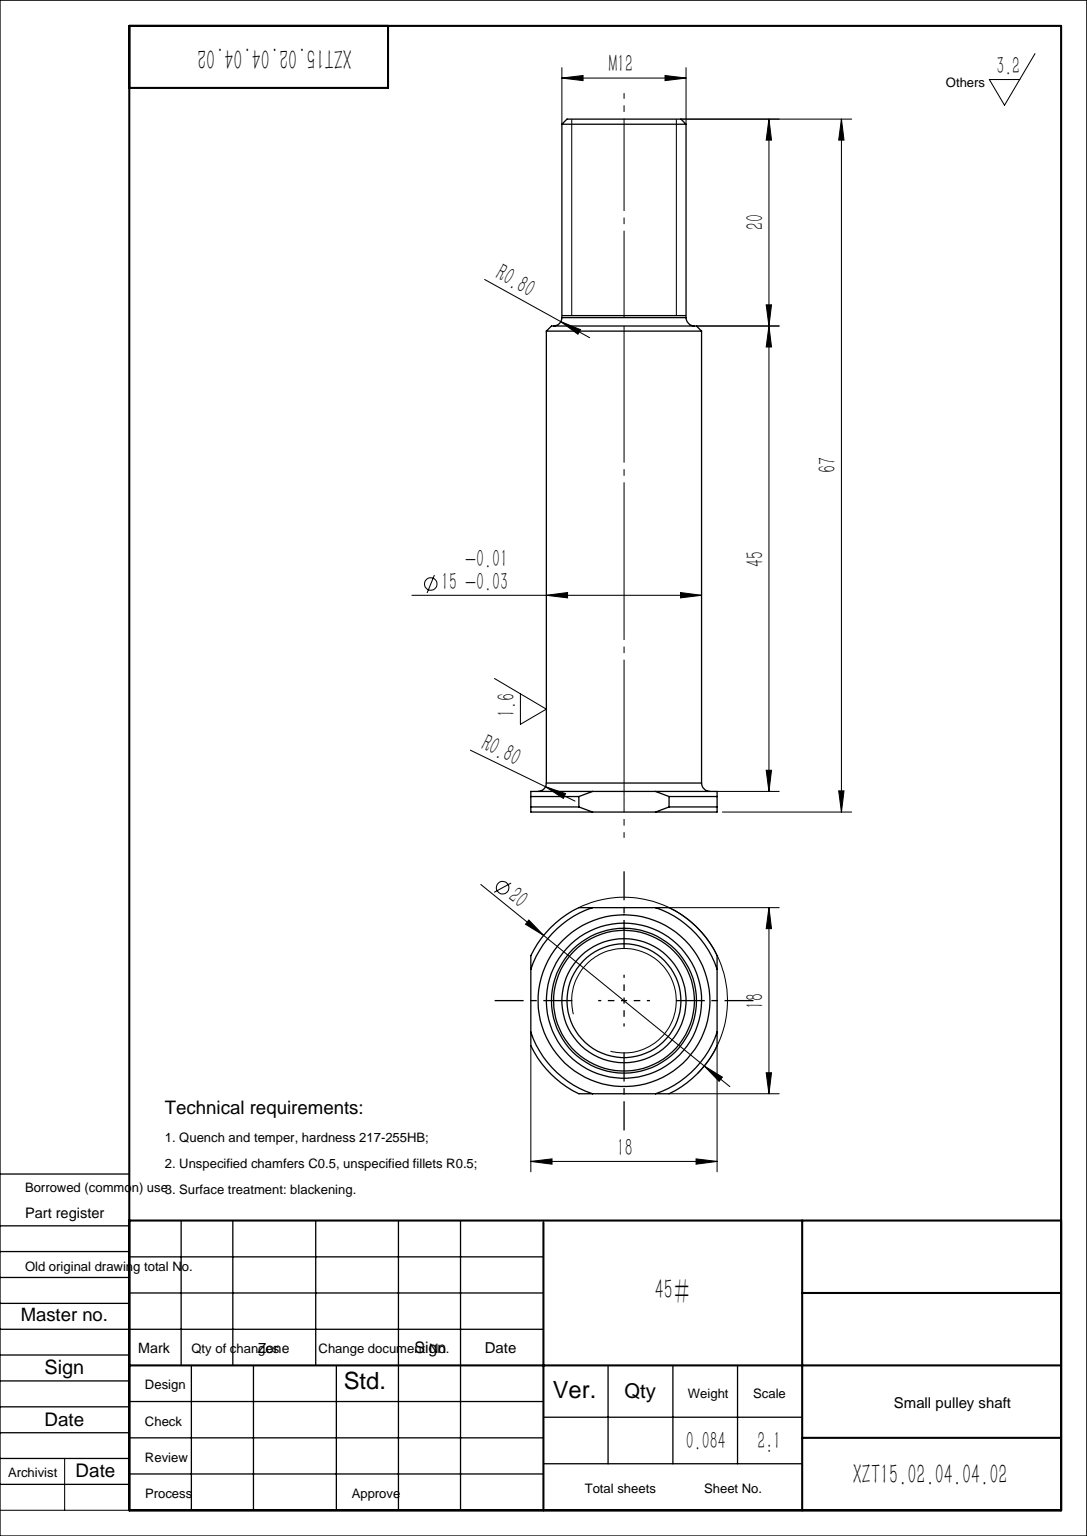
from build123d import *

# Parameters (mm, degrees)
CHAMFER1_SIZE       = 0.5
FILLET1_R           = 0.8
SKETCH2_OUTSIDE_W   = 36.546
SKETCH2_OUTSIDE_H   = 36.546
SKETCH2_OUTSIDE_W_2 = 18
SKETCH2_OUTSIDE_H_2 = 18
CUT_EXTRUDE1_DEPTH  = 10


with BuildPart() as part:
    # Sketch1 → Revolve1 (revolve)
    with BuildSketch(Plane.XY, mode=Mode.PRIVATE) as revolve1_sk:
        Polygon((0, 0), (10, 0), (10, 2), (7.5, 2), (7.5, 47), (6, 47), (6, 67), (0, 67), align=None)
    revolve(revolve1_sk.sketch.rotate(Axis((0, 0, 0), (0, -1, 0)), 90), axis=Axis((0, 0, 0), (0, -1, 0)))

    # Chamfer1
    chamfer1_edges = [part.edges().sort_by_distance(p)[0] for p in [
        (0, 67, -6),
        (0, 47, -7.5),
        (0, 2, -10),
        (0, 0, -10),
    ]]
    chamfer(chamfer1_edges, length=CHAMFER1_SIZE)

    # Fillet1
    fillet1_edges = [part.edges().sort_by_distance(p)[0] for p in [
        (0, 47, -6),
        (0, 2, -7.5),
    ]]
    fillet(fillet1_edges, radius=FILLET1_R)

    # Sketch2 outside → Cut-Extrude1 (cut)
    with BuildSketch(Plane(origin=(0, 0, 0), x_dir=(1, 0, 0), z_dir=(0, 1, 0))):
        Rectangle(SKETCH2_OUTSIDE_W, SKETCH2_OUTSIDE_H)
        Rectangle(SKETCH2_OUTSIDE_W_2, SKETCH2_OUTSIDE_H_2, mode=Mode.SUBTRACT)
    extrude(amount=CUT_EXTRUDE1_DEPTH, mode=Mode.SUBTRACT)


solid = part.part
